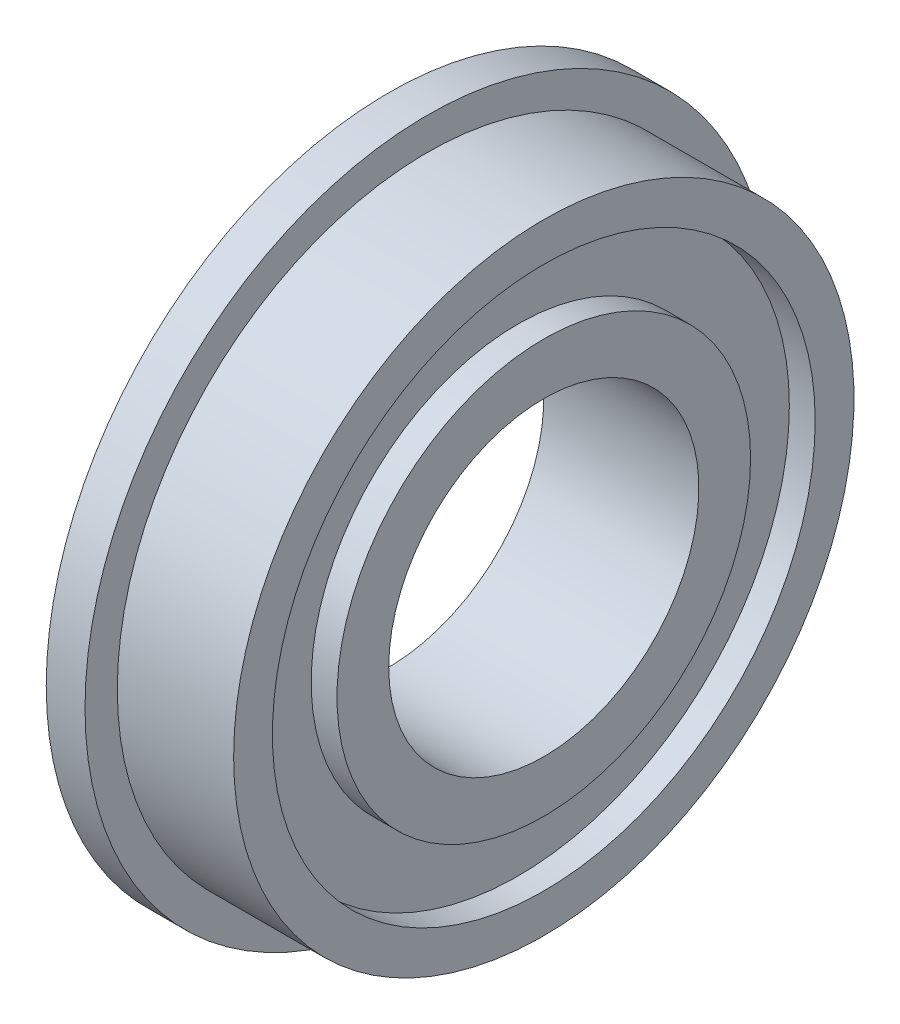
from build123d import *

# Parameters (mm, degrees)
SKETCH2_R          = 10.5
SKETCH2_R_2        = 8
CUT_EXTRUDE1_DEPTH = 1
CUT_EXTRUDE2_START = -1
SKETCH3_R          = 10.5
SKETCH3_R_2        = 8
CUT_EXTRUDE2_DEPTH = 1


with BuildPart() as part:
    # Sketch1 → Revolve1 (revolve)
    with BuildSketch(Plane.XY, mode=Mode.PRIVATE) as revolve1_sk:
        Polygon((0, 6), (6, 6), (6, 12), (1.5, 12), (1.5, 13.25), (0, 13.25), align=None)
    revolve(revolve1_sk.sketch.rotate(Axis((0, 0, 0), (1, 0, 0)), 90), axis=Axis((0, 0, 0), (1, 0, 0)))

    # Sketch2 → Cut-Extrude1 (cut)
    with BuildSketch(Plane(origin=(6, 0, 0), x_dir=(0, 0, -1), z_dir=(1, 0, 0))):
        Circle(SKETCH2_R)
        Circle(SKETCH2_R_2, mode=Mode.SUBTRACT)
    extrude(amount=-CUT_EXTRUDE1_DEPTH, mode=Mode.SUBTRACT)

    # Sketch3 → Cut-Extrude2 (cut)
    with BuildSketch(Plane.ZY.offset(CUT_EXTRUDE2_START)):
        with Locations(Location((0, 0, 0), (0, 0, 180))):
            Circle(SKETCH3_R)
        with Locations(Location((0, 0, 0), (0, 0, 180))):
            Circle(SKETCH3_R_2, mode=Mode.SUBTRACT)
    extrude(amount=CUT_EXTRUDE2_DEPTH, mode=Mode.SUBTRACT)


solid = part.part
